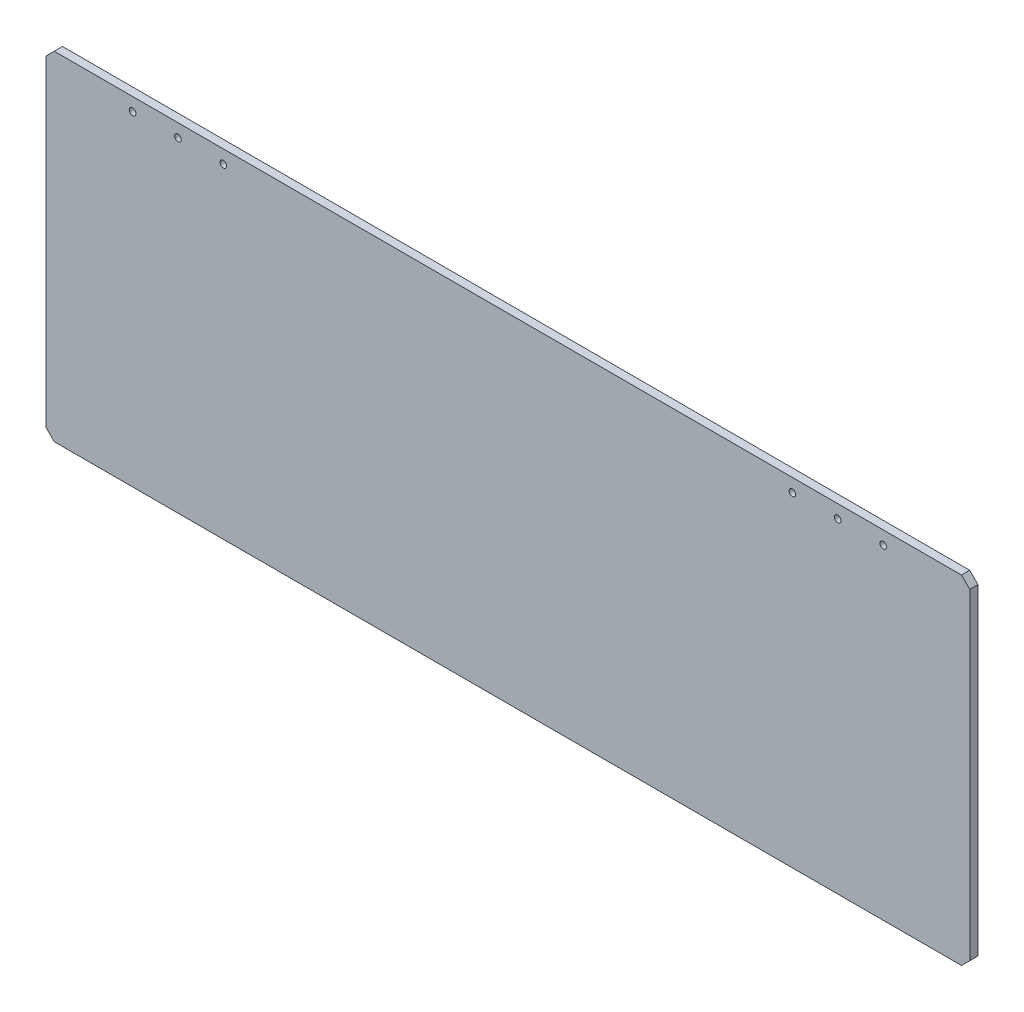
from build123d import *

# Parameters (mm, degrees)
SKETCH1_R           = 2
BOSS_EXTRUDE1_DEPTH = 5


with BuildPart() as part:
    # Sketch1 → Boss-Extrude1 (new body)
    with BuildSketch(Plane.XY):
        Polygon((0, -5), (5, 0), (555, 0), (560, -5), (560, -200), (555, -205), (5, -205), (0, -200), align=None)
        with Locations((52.5, -8)):
            Circle(SKETCH1_R, mode=Mode.SUBTRACT)
        with Locations((80, -8)):
            Circle(SKETCH1_R, mode=Mode.SUBTRACT)
        with Locations((107.5, -8)):
            Circle(SKETCH1_R, mode=Mode.SUBTRACT)
        with Locations(Location((452.5, -8, 0), (0, 0, 180))):
            Circle(SKETCH1_R, mode=Mode.SUBTRACT)
        with Locations(Location((480, -8, 0), (0, 0, 180))):
            Circle(SKETCH1_R, mode=Mode.SUBTRACT)
        with Locations(Location((507.5, -8, 0), (0, 0, 180))):
            Circle(SKETCH1_R, mode=Mode.SUBTRACT)
    extrude(amount=BOSS_EXTRUDE1_DEPTH)


solid = part.part
